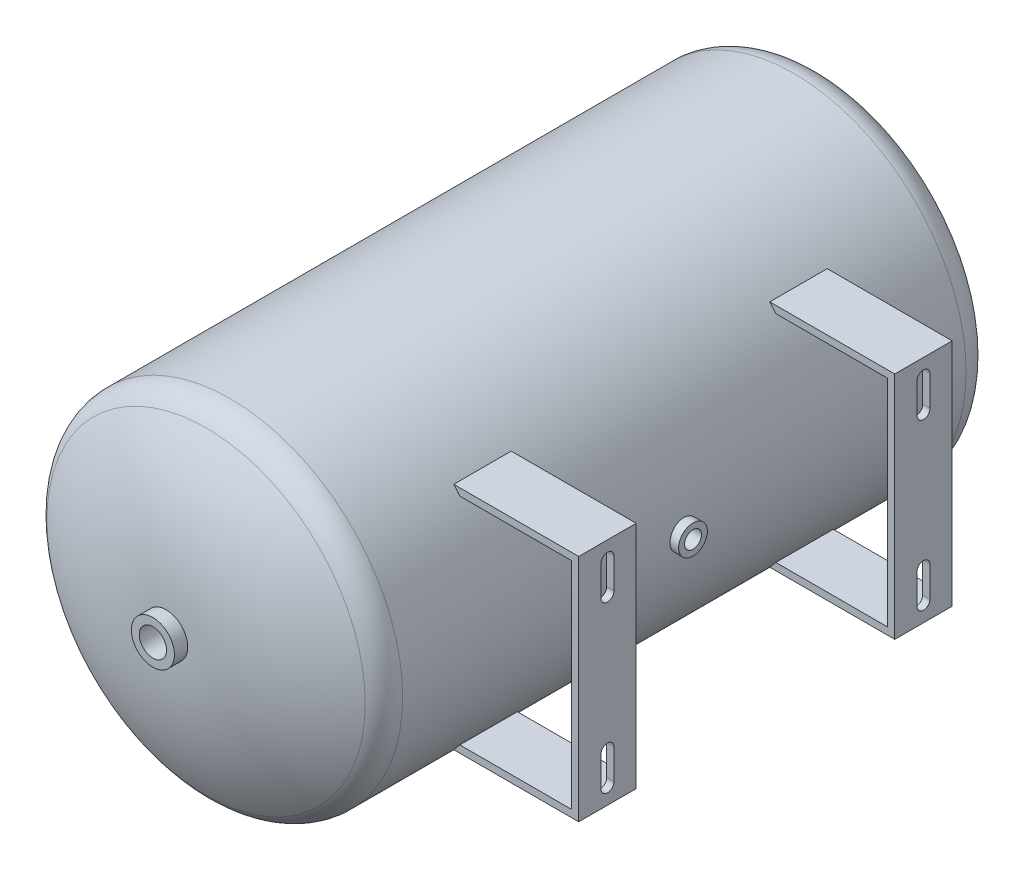
from build123d import *

# Parameters (mm, degrees)
SKETCH_1_R               = 120
EXTRUDE_1_DEPTH          = 180
EXTRUDE_2_DEPTH          = 20
CUT_EXTRUDE_1_DEPTH      = 6
SKETCH_17_R              = 15
EXTRUDE_3_DEPTH          = 20
HOLE_WIZARD_G1_2_1_D     = 19
HOLE_WIZARD_G1_2_1_DEPTH = 30
HOLE_WIZARD_G1_2_1_TIP   = 5.708175881
SKETCH_20_R              = 15
EXTRUDE_4_DEPTH          = 15
HOLE_WIZARD_G1_2_2_D     = 19
HOLE_WIZARD_G1_2_2_DEPTH = 47.35
HOLE_WIZARD_G1_2_2_TIP   = 5.708175881
HOLE_WIZARD_G1_2_3_D     = 19
HOLE_WIZARD_G1_2_3_DEPTH = 47.35
HOLE_WIZARD_G1_2_3_TIP   = 5.708175881
SKETCH_26_R              = 10
EXTRUDE_5_DEPTH          = 16
HOLE_WIZARD_G1_4_1_D     = 11.8
HOLE_WIZARD_G1_4_1_DEPTH = 30.32
HOLE_WIZARD_G1_4_1_TIP   = 3.545077652


with BuildPart() as part:
    # 草图1 → 凸台-拉伸1 (new, symmetric)
    with BuildSketch(Plane.XY):
        with Locations(Location((0, 0, 0), (0, 0, 180))):
            Circle(SKETCH_1_R)
    extrude(amount=EXTRUDE_1_DEPTH, both=True)

    # 草图2 → 旋转1 (revolve)
    with BuildSketch(Plane(origin=(0, 0, 0), x_dir=(1, 0, 0), z_dir=(0, 1, 0)), mode=Mode.PRIVATE) as revolve_1_sk:
        with BuildLine():
            Line((0, 180), (120, 180))
            Line((120, 180), (120, 196.124178579))
            ThreePointArc((120, 196.124178579), (117.549645232, 205.716360408), (110.799004776, 212.958117388))
            ThreePointArc((110.799004776, 212.958117388), (57.657842502, 235.732180627), (0, 240))
            Line((0, 240), (0, 180))
        make_face()
    revolve_1 = revolve(revolve_1_sk.sketch.rotate(Axis((0, 0, -180), (0, 0, 1)), 180), axis=Axis((0, 0, -180), (0, 0, 1)))

    # 镜向1: 旋转1 across plane
    add(revolve_1.mirror(Plane.XY))

    # 草图15 → 凸台-拉伸2 (add, symmetric)
    with BuildSketch(Plane.XY.offset(110)):
        with BuildLine():
            Line((93.674969976, -75), (171.4427191, -75))
            Line((171.4427191, -75), (171.4427191, 75))
            Line((171.4427191, 75), (93.674969976, 75))
            ThreePointArc((93.674969976, 75), (91.592969234, 77.528884855), (89.4427191, 80))
            Line((89.4427191, 80), (176.4427191, 80))
            Line((176.4427191, 80), (176.4427191, -80))
            Line((176.4427191, -80), (89.4427191, -80))
            ThreePointArc((89.4427191, -80), (91.592969234, -77.528884855), (93.674969976, -75))
        make_face()
    extrude_2 = extrude(amount=EXTRUDE_2_DEPTH, both=True)

    # 镜向2: 凸台-拉伸2 across plane
    add(extrude_2.mirror(Plane.XY))

    # 草图16 → 切除-拉伸1 (cut)
    with BuildSketch(Plane(origin=(176.4427191, 0, 0), x_dir=(0, 0, -1), z_dir=(1, 0, 0))):
        with BuildLine():
            Line((-105.5, 68), (-105.5, 47))
            ThreePointArc((-105.5, 47), (-110, 42.5), (-114.5, 47))
            Line((-114.5, 47), (-114.5, 68))
            ThreePointArc((-114.5, 68), (-110, 72.5), (-105.5, 68))
        make_face()
        with BuildLine():
            Line((-114.5, -68), (-114.5, -47))
            ThreePointArc((-114.5, -47), (-110, -42.5), (-105.5, -47))
            Line((-105.5, -47), (-105.5, -68))
            ThreePointArc((-105.5, -68), (-110, -72.5), (-114.5, -68))
        make_face()
        with BuildLine():
            Line((105.5, 68), (105.5, 47))
            ThreePointArc((105.5, 47), (110, 42.5), (114.5, 47))
            Line((114.5, 47), (114.5, 68))
            ThreePointArc((114.5, 68), (110, 72.5), (105.5, 68))
        make_face()
        with BuildLine():
            Line((114.5, -68), (114.5, -47))
            ThreePointArc((114.5, -47), (110, -42.5), (105.5, -47))
            Line((105.5, -47), (105.5, -68))
            ThreePointArc((105.5, -68), (110, -72.5), (114.5, -68))
        make_face()
    extrude(amount=-CUT_EXTRUDE_1_DEPTH, mode=Mode.SUBTRACT)

    # 草图17 → 凸台-拉伸3 (add)
    with BuildSketch(Plane(origin=(-110, 0, 0), x_dir=(0, 0, -1), z_dir=(1, 0, 0))):
        Circle(SKETCH_17_R)
        with Locations((100, 0)):
            Circle(SKETCH_17_R)
        with Locations((-100, 0)):
            Circle(SKETCH_17_R)
    extrude(amount=-EXTRUDE_3_DEPTH)

    # G1/2 螺纹孔1
    with Locations(Plane.ZY.offset(130)):
        with Locations((-100, 0), (0, 0), (100, 0)):
            Hole(HOLE_WIZARD_G1_2_1_D / 2, depth=HOLE_WIZARD_G1_2_1_DEPTH)
            with Locations((0, 0, -(HOLE_WIZARD_G1_2_1_DEPTH + HOLE_WIZARD_G1_2_1_TIP / 2))):  # 118° drill point
                Cone(0, HOLE_WIZARD_G1_2_1_D / 2, HOLE_WIZARD_G1_2_1_TIP, mode=Mode.SUBTRACT)

    # 草图20 → 凸台-拉伸4 (add)
    with BuildSketch(Plane.XY.offset(235)):
        with Locations(Location((0, 0, 0), (0, 0, 180))):
            Circle(SKETCH_20_R)
    extrude_4 = extrude(amount=EXTRUDE_4_DEPTH)

    # G1/2 螺纹孔2
    with Locations(Plane.XY.offset(250)):
        with Locations((0, 0)):
            Hole(HOLE_WIZARD_G1_2_2_D / 2, depth=HOLE_WIZARD_G1_2_2_DEPTH)
            with Locations((0, 0, -(HOLE_WIZARD_G1_2_2_DEPTH + HOLE_WIZARD_G1_2_2_TIP / 2))):  # 118° drill point
                Cone(0, HOLE_WIZARD_G1_2_2_D / 2, HOLE_WIZARD_G1_2_2_TIP, mode=Mode.SUBTRACT)

    # 镜向3: 凸台-拉伸4 across plane
    add(extrude_4.mirror(Plane.XY))

    # G1/2 螺纹孔3
    with Locations(Plane(origin=(0, 0, -250), x_dir=(-1, 0, 0), z_dir=(0, 0, -1))):
        with Locations((0, 0)):
            Hole(HOLE_WIZARD_G1_2_3_D / 2, depth=HOLE_WIZARD_G1_2_3_DEPTH)
            with Locations((0, 0, -(HOLE_WIZARD_G1_2_3_DEPTH + HOLE_WIZARD_G1_2_3_TIP / 2))):  # 118° drill point
                Cone(0, HOLE_WIZARD_G1_2_3_D / 2, HOLE_WIZARD_G1_2_3_TIP, mode=Mode.SUBTRACT)

    # 草图26 → 凸台-拉伸5 (add)
    with BuildSketch(Plane(origin=(110, 0, 0), x_dir=(0, 0, -1), z_dir=(1, 0, 0))):
        with Locations(Location((0, 0, 0), (0, 0, 180))):
            Circle(SKETCH_26_R)
    extrude(amount=EXTRUDE_5_DEPTH)

    # G1/4 螺纹孔1
    with Locations(Plane(origin=(126, 0, 0), x_dir=(0, 0, -1), z_dir=(1, 0, 0))):
        with Locations((0, 0)):
            Hole(HOLE_WIZARD_G1_4_1_D / 2, depth=HOLE_WIZARD_G1_4_1_DEPTH)
            with Locations((0, 0, -(HOLE_WIZARD_G1_4_1_DEPTH + HOLE_WIZARD_G1_4_1_TIP / 2))):  # 118° drill point
                Cone(0, HOLE_WIZARD_G1_4_1_D / 2, HOLE_WIZARD_G1_4_1_TIP, mode=Mode.SUBTRACT)


solid = part.part
